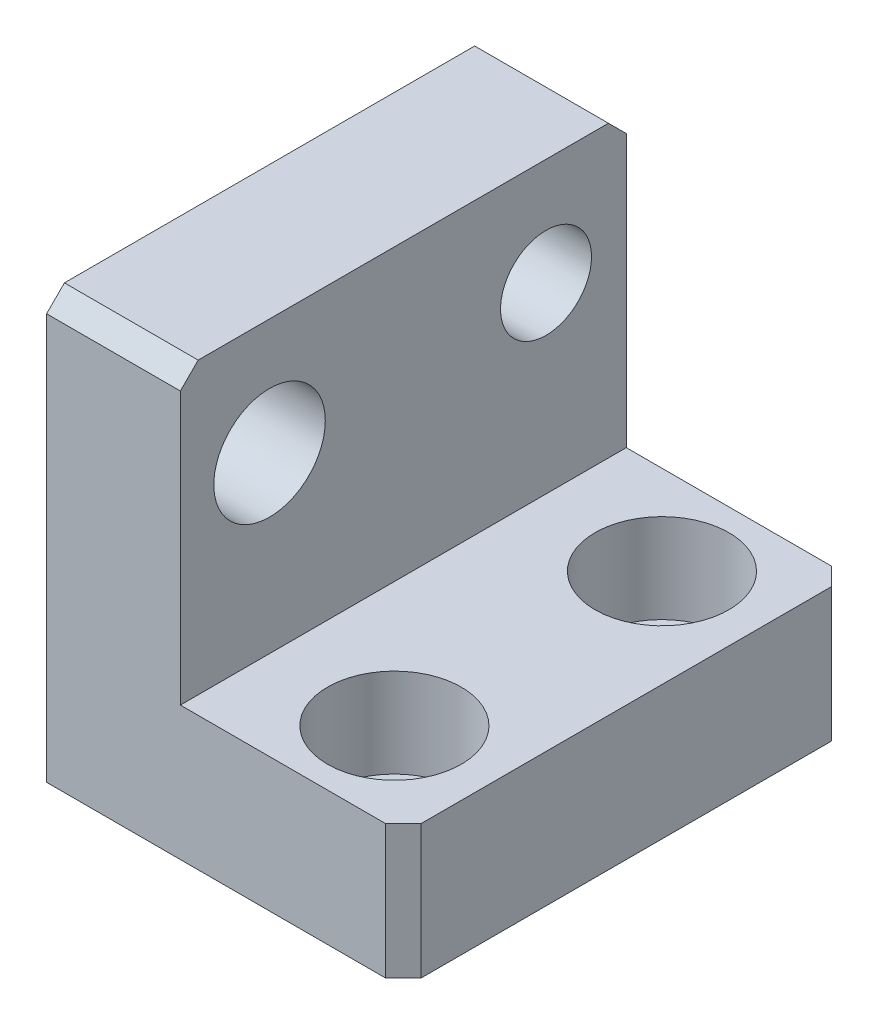
from build123d import *

# Parameters (mm, degrees)
BOSS_EXTRUDE1_DEPTH    = 50
CHAMFER2_SIZE          = 2
HOLE4_D                = 9
HOLE4_CBORE_D          = 15
HOLE4_CBORE_DEPTH      = 10
M14X1_5_TAPPED_HOLE1_D = 12.5
M12_TAPPED_HOLE1_D     = 10.2


with BuildPart() as part:
    # Sketch1 → Boss-Extrude1 (new body)
    with BuildSketch(Plane.XY):
        Polygon((-40.819758101, 19.90625), (-40.819758101, -27.59375), (-0.819758101, -27.59375), (-0.819758101, -12.59375), (-25.819758101, -12.59375), (-25.819758101, 19.90625), align=None)
    extrude(amount=BOSS_EXTRUDE1_DEPTH)

    # Chamfer2
    chamfer2_edges = [part.edges().sort_by_distance(p)[0] for p in [
        (-0.819758101, -20.09375, 50),
        (-33.319758101, 19.90625, 50),
        (-0.819758101, -20.09375, 0),
        (-33.319758101, 19.90625, 0),
    ]]
    chamfer(chamfer2_edges, length=CHAMFER2_SIZE)

    # Hole4 (through all)
    with Locations(Plane(origin=(0, -12.59375, 0), x_dir=(1, 0, 0), z_dir=(0, 1, 0))):
        with Locations((-11.819758101, -10), (-11.819758101, -40)):
            CounterBoreHole(HOLE4_D / 2, HOLE4_CBORE_D / 2, HOLE4_CBORE_DEPTH)

    # M14x1.5 Tapped Hole1 (through all)
    with Locations(Plane(origin=(-25.819758101, 0, 0), x_dir=(0, 0, -1), z_dir=(1, 0, 0))):
        with Locations((-40, 6.90625)):
            Hole(M14X1_5_TAPPED_HOLE1_D / 2)

    # M12 Tapped Hole1 (through all)
    with Locations(Plane(origin=(-25.819758101, 0, 0), x_dir=(0, 0, -1), z_dir=(1, 0, 0))):
        with Locations((-9, 7.90625)):
            Hole(M12_TAPPED_HOLE1_D / 2)


solid = part.part
